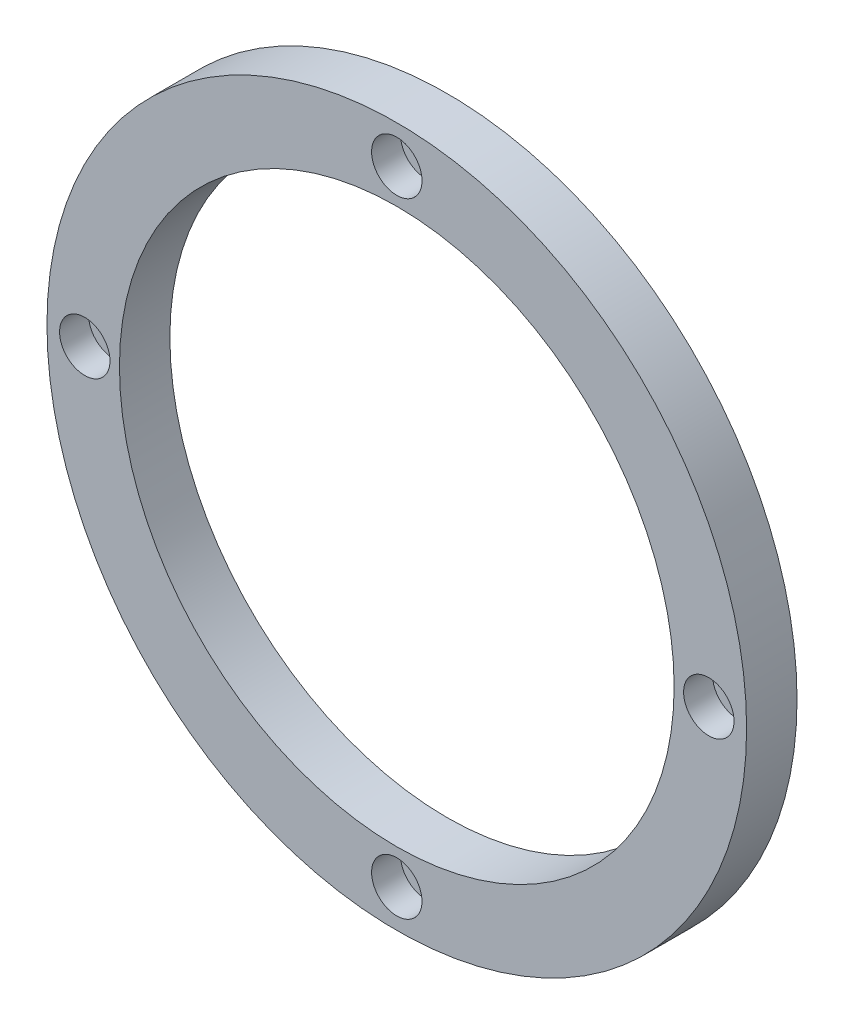
SolidWorks part; units mm, degrees
ref_plane "Front Plane" through (0, 0, 0) normal (0, 0, 1) x (1, 0, 0)
ref_plane "Top Plane" through (0, 0, 0) normal (0, 1, 0) x (1, 0, 0)
ref_plane "Right Plane" through (0, 0, 0) normal (1, 0, 0) x (0, 0, -1)
sketch "Sketch1" plane through (0, 0, 0) normal (0, 0, 1) x (1, 0, 0)
  circle A0 centre (0, 0) radius 44
  circle A1 centre (0, 0) radius 55.5
  dimension "D1" = 111
  dimension "D2" = 88
extrude "Boss-Extrude1" add sketch "Sketch1" along normal blind 8
hole_wizard "Hole size per socket head cap screw type 1" positions "Sketch4" profile "Sketch5" counterbore size "M4" standard "GB"
sketch "Sketch4" plane through (0, 0, 8) normal (0, 0, 1) x (1, 0, 0)
  circle A0 centre (0, 0) radius 49.5 construction
  point P0 (0, 49.5)
  dimension "D1" = 99
sketch "Sketch5" plane through (0, 49.5, 8) normal (1, 0, 0) x (0, -1, 0)
  line L0 (0, 0) -> (0, 18.3519)
  line L1 (0, 18.3519) -> (2.25, 17)
  line L2 (2.25, 17) -> (2.25, 4.6)
  line L3 (2.25, 4.6) -> (4, 4.6)
  line L4 (4, 4.6) -> (4, 0)
  line L5 (4, 0) -> (0, 0)
  line L10 (0, 18.3519) -> (-2.25, 17) construction
  line L11 (0, -6.35) -> (0, 107.95) construction
  dimension "孔直径" = 4.5
  dimension "孔深度" = 17
  dimension "柱形沉头孔直径" = 8
  dimension "柱形沉头孔深度" = 4.6
  dimension "导头角度" = 118
pattern_circular "CirPattern1" count 4 over 360 about axis through (0, 0, 0) along (0, 0, 1) of "Hole size per socket head cap screw type 1"
